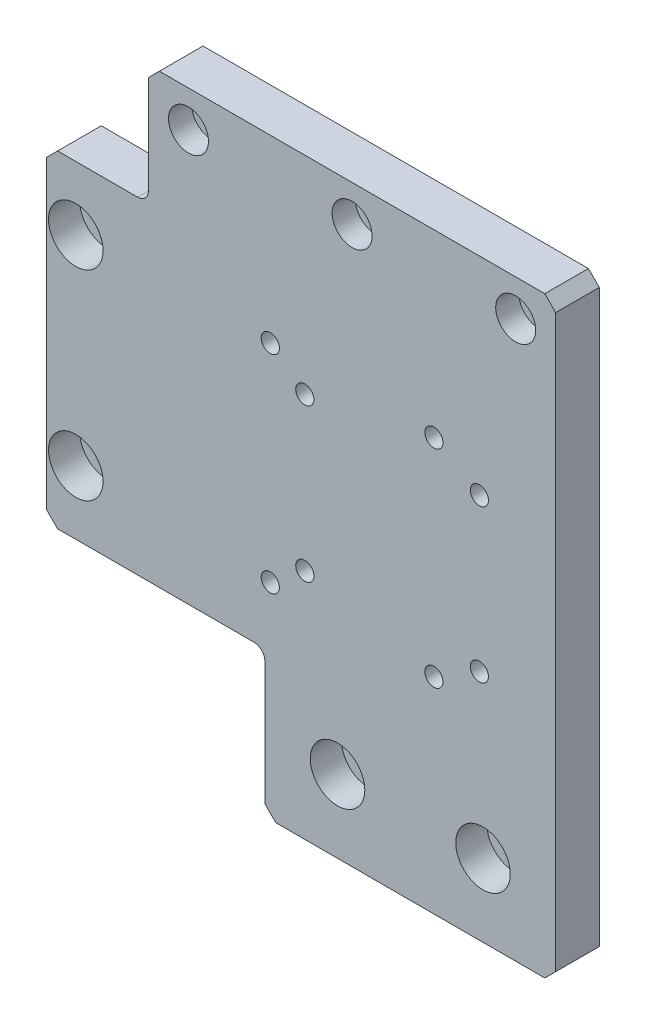
from build123d import *

# Parameters (mm, degrees)
SKETCH_1_W                     = 140
SKETCH_1_H                     = 112
EXTRUDE_1_DEPTH                = 12
HOLE_WIZARD_M6_1_D             = 5
HOLE_WIZARD_M6_2_D             = 5
SKETCH_6_W                     = 112
SKETCH_6_H                     = 12
EXTRUDE_2_DEPTH                = 22
SKETCH_7_W                     = 28
SKETCH_7_H                     = 12
CUT_EXTRUDE_1_DEPTH            = 11
SKETCH_8_W                     = 60
SKETCH_8_H                     = 12
CUT_EXTRUDE_2_DEPTH            = 11
HOLE_WIZARD_M6_1_2_D           = 6.6
HOLE_WIZARD_M6_1_2_CBORE_D     = 11
HOLE_WIZARD_M6_1_2_CBORE_DEPTH = 6.4
SKETCH_11_W                    = 80
SKETCH_11_H                    = 12
EXTRUDE_3_DEPTH                = 29
CHAMFER_1_SIZE                 = 3
FILLET_1_R                     = 3
HOLE_WIZARD_M8_1_D             = 9
HOLE_WIZARD_M8_1_CBORE_D       = 15
HOLE_WIZARD_M8_1_CBORE_DEPTH   = 8.6
HOLE_WIZARD_M8_2_D             = 9
HOLE_WIZARD_M8_2_CBORE_D       = 15
HOLE_WIZARD_M8_2_CBORE_DEPTH   = 8.6


with BuildPart() as part:
    # 草图1 → 凸台-拉伸1 (new body)
    with BuildSketch(Plane.XY):
        with Locations((70, 56)):
            Rectangle(SKETCH_1_W, SKETCH_1_H)
    extrude(amount=EXTRUDE_1_DEPTH)

    # Hole Wizard M6 _1 (through all)
    with Locations(Plane(origin=(0, 0, 0), x_dir=(-1, 0, 0), z_dir=(0, 0, -1))):
        with Locations((-106.5, 84.5), (-61.5, 84.5), (-61.5, 27.5), (-106.5, 27.5)):
            Hole(HOLE_WIZARD_M6_1_D / 2)

    # M6 螺纹孔2 (through all)
    with Locations(Plane.XY.offset(12)):
        with Locations((71, 77), (71, 35), (119, 35), (119, 77)):
            Hole(HOLE_WIZARD_M6_2_D / 2)

    # 草图6 → 凸台-拉伸2 (add)
    with BuildSketch(Plane(origin=(0, 112, 0), x_dir=(1, 0, 0), z_dir=(0, 1, 0))):
        with Locations((84, -6)):
            Rectangle(SKETCH_6_W, SKETCH_6_H)
    extrude(amount=EXTRUDE_2_DEPTH)

    # 草图7 → 切除-拉伸1 (cut)
    with BuildSketch(Plane(origin=(0, 112, 0), x_dir=(1, 0, 0), z_dir=(0, 1, 0))):
        with Locations((14, -6)):
            Rectangle(SKETCH_7_W, SKETCH_7_H)
    extrude(amount=-CUT_EXTRUDE_1_DEPTH, mode=Mode.SUBTRACT)

    # 草图8 → 切除-拉伸2 (cut)
    with BuildSketch(Plane.XZ):
        with Locations((30, 6)):
            Rectangle(SKETCH_8_W, SKETCH_8_H)
    extrude(amount=-CUT_EXTRUDE_2_DEPTH, mode=Mode.SUBTRACT)

    # Hole Wizard M6 _1 2 (through all)
    with Locations(Plane.XY.offset(12)):
        with Locations((129, 124), (84, 124), (39, 124)):
            CounterBoreHole(HOLE_WIZARD_M6_1_2_D / 2, HOLE_WIZARD_M6_1_2_CBORE_D / 2, HOLE_WIZARD_M6_1_2_CBORE_DEPTH)

    # 草图11 → 凸台-拉伸3 (add)
    with BuildSketch(Plane.XZ):
        with Locations((100, 6)):
            Rectangle(SKETCH_11_W, SKETCH_11_H)
    extrude(amount=EXTRUDE_3_DEPTH)

    # 倒角1
    chamfer_1_edges = [part.edges().sort_by_distance(p)[0] for p in [
        (140, -29, 6),
        (60, -29, 6),
        (0, 11, 6),
        (140, 134, 6),
        (0, 101, 6),
        (28, 134, 6),
    ]]
    chamfer(chamfer_1_edges, length=CHAMFER_1_SIZE)

    # 圆角1
    fillet_1_edges = [part.edges().sort_by_distance(p)[0] for p in [
        (28, 101, 6),
        (60, 11, 6),
    ]]
    fillet(fillet_1_edges, radius=FILLET_1_R)

    # M8 六角凹头螺钉的柱形沉头孔1 (through all)
    with Locations(Plane.XY.offset(12)):
        with Locations((8, 83.5), (8, 28.5)):
            CounterBoreHole(HOLE_WIZARD_M8_1_D / 2, HOLE_WIZARD_M8_1_CBORE_D / 2, HOLE_WIZARD_M8_1_CBORE_DEPTH)

    # M8 六角凹头螺钉的柱形沉头孔2 (through all)
    with Locations(Plane.XY.offset(12)):
        with Locations((80, -9), (120, -9)):
            CounterBoreHole(HOLE_WIZARD_M8_2_D / 2, HOLE_WIZARD_M8_2_CBORE_D / 2, HOLE_WIZARD_M8_2_CBORE_DEPTH)


solid = part.part
